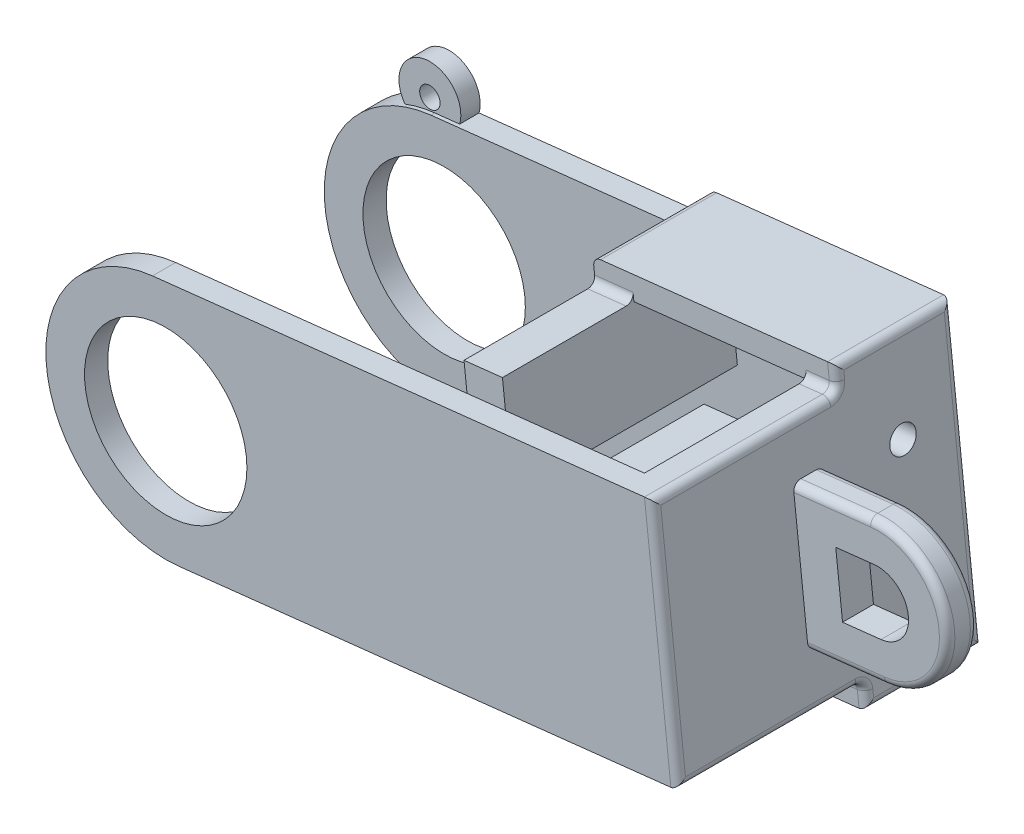
SolidWorks part; units mm, degrees
ref_plane "Front Plane" through (0, 0, 0) normal (0, 0, 1) x (1, 0, 0)
ref_plane "Top Plane" through (0, 0, 0) normal (0, 1, 0) x (1, 0, 0)
ref_plane "Right Plane" through (0, 0, 0) normal (1, 0, 0) x (0, 0, -1)
sketch "Sketch1" plane through (0, 0, 0) normal (0, 0, 1) x (1, 0, 0)
  line L0 (132.6238, -16.4902) -> (3.415, -30.8113)
  line L1 (132.6238, -16.4902) -> (125.7937, 45.1325)
  line L3 (125.7937, 45.1325) -> (-3.415, 30.8113)
  line L8 (33.2276, 36.08) -> (-40.322, 27.928) construction
  circle A0 centre (0, 0) radius 21
  arc A1 (-3.415, 30.8113) -> (3.415, -30.8113) centre (0, 0) ccw
  point P5 (71.547, -23.7484)
  dimension "D1" = 42
  dimension "D2" = 62
  dimension "D3" = 130
  dimension "D4" = 62
extrude "Boss-Extrude1" add sketch "Sketch1" against normal blind 6
sketch "Sketch2" plane through (0, 0, 0) normal (0, 0, 1) x (1, 0, 0)
  line L0 (125.7937, 45.1325) -> (132.6238, -16.4902)
  line L5 (132.6238, -16.4902) -> (125.7937, 45.1325) construction
  line L6 (132.6238, -16.4902) -> (124.6276, -17.3765)
  line L7 (3.415, -30.8113) -> (132.6238, -16.4902) construction
  line L8 (124.6276, -17.3765) -> (117.7975, 44.2462)
  line L9 (117.7975, 44.2462) -> (125.7937, 45.1325)
  dimension "D1" = 7.9962
extrude "Boss-Extrude2" add sketch "Sketch2" against normal blind 78
ref_plane "Plane1" through (0, 0, -39) normal (0, 0, 1) x (1, 0, 0)
sketch "Sketch3" plane through (0, 0, -6) normal (0, 0, -1) x (-1, 0, 0)
  circle A0 centre (-50, 5.8897) radius 3
  circle A1 centre (0, 0) radius 12.5 construction
  dimension "D1" = 6
  dimension "D2" = 50
extrude "Boss-Extrude3" add sketch "Sketch3" along normal blind 28
sketch "Sketch4" plane through (0, 0, -6) normal (0, 0, -1) x (-1, 0, 0)
  line L0 (-73.0714, 39.2889) -> (-79.9015, -22.3338)
  line L1 (-125.7937, 45.1325) -> (-117.7975, 44.2462) construction
  line L2 (-124.6276, -17.3765) -> (-132.6238, -16.4902) construction
  line L3 (-79.9015, -22.3338) -> (-69.9624, -23.4354)
  line L4 (-69.9624, -23.4354) -> (-63.1323, 38.1872)
  line L5 (-63.1323, 38.1872) -> (-73.0714, 39.2889)
  line L6 (-117.7975, 44.2462) -> (-124.6276, -17.3765) construction
  dimension "D1" = 10
  dimension "D2" = 45
extrude "Boss-Extrude4" add sketch "Sketch4" along normal blind 71
sketch "Sketch10" plane through (0, 0, -34) normal (0, 0, -1) x (-1, 0, 0)
  circle A0 centre (-50, 5.8897) radius 4
extrude "Boss-Extrude6" add sketch "Sketch10" against normal blind 1
mirror "Mirror1" about plane through (0, 0, -39) normal (0, 0, 1) of bodies 119 107
sketch "Sketch6" plane through (0, 0, -6) normal (0, 0, -1) x (-1, 0, 0)
  line L0 (-77.7989, 39.8128) -> (-50.5325, 36.7907)
  line L1 (-117.7975, 44.2462) -> (-73.0714, 39.2889) construction
  line L2 (-63.1323, 38.1872) -> (3.415, 30.8113) construction
  line L3 (-50.5325, 36.7907) -> (-51.8362, 25.0286)
  line L4 (-51.8362, 25.0286) -> (-77.7989, 27.9062)
  line L5 (-77.7989, 27.9062) -> (-77.7989, 39.8128)
extrude "Cut-Extrude1" cut sketch "Sketch6" along normal blind 8
ref_plane "Plane2" through (0, 0, 0) normal (-0.1102, 0.9939, 0) x (0.9939, 0.1102, 0)
mirror "Mirror4" about plane through (0, 0, 0) normal (-0.1102, 0.9939, 0) of "Cut-Extrude1"
sketch "Sketch8" plane through (66.5473, 7.3759, 0) normal (-0.9939, -0.1102, 0) x (0, 0, 1)
  line L0 (-72, -31) -> (-72, 31) construction
  line L1 (-72, 0) -> (-6, 0)
  line L2 (-72, 0) -> (-72, 6)
  line L3 (-72, 6) -> (-6, 6)
  line L4 (-6, 0) -> (-6, 6)
  line L5 (-6, 31) -> (-6, -31) construction
  dimension "D1" = 6
extrude "Cut-Extrude3" cut sketch "Sketch8" against normal blind 15
mirror "Mirror5" about plane through (81.456, 9.0284, -72) normal (0.1102, -0.9939, 0) of "Cut-Extrude3"
sketch "Sketch11" plane through (-3.415, 30.8113, 0) normal (-0.1102, 0.9939, 0) x (0.9939, 0.1102, 0)
  line L0 (66.9548, 72) -> (66.9548, 14) construction
  line L1 (130, 78) -> (66.9548, 78)
  line L2 (130, 78) -> (130, 48)
  line L3 (130, 48) -> (66.9548, 48)
  line L4 (66.9548, 78) -> (66.9548, 48)
  dimension "D1" = 30
extrude "Boss-Extrude7" add sketch "Sketch11" along normal blind 6
mirror "Mirror6" about plane through (0, 0, 0) normal (-0.1102, 0.9939, 0) of "Boss-Extrude7"
fillet "Fillet2" radius 2 14 edges at (125.7937, 45.1325, -24) (125.4632, 48.1142, -48) (125.1328, 51.0959, -63) (129.2088, 14.3211, -78) (133.2848, -22.4537, -63) (132.9543, -19.4719, -48) (132.6238, -16.4902, -24) (129.2088, 14.3211, 0) (70.6233, -29.3989, -63) (62.4713, 44.1507, -63) (68.1019, 38.7381, -48) (121.7956, 44.6893, -48) (74.9319, -22.8846, -48) (128.6257, -16.9333, -48)
sketch "Sketch12" plane through (129.2088, 14.3211, 0) normal (0.9939, 0.1102, 0) x (0, 0, -1)
  line L0 (50, -35) -> (76, -35) construction
  circle A0 centre (63, 14) radius 6.3103
  circle A1 centre (63, -16) radius 7.3998
  point P0 (63, 14)
  point P2 (63, -16)
  dimension "D1" = 30
  dimension "D2" = 19
hole_wizard "Tap Drill for M8 Tap1" positions "Sketch12" profile "Sketch13" hole size "M8" standard "GB"
sketch "Sketch13" plane through (127.6665, 28.2359, -63) normal (0, 0, 1) x (-0.1102, 0.9939, 0)
  line L0 (0, 0) -> (0, 22.0429)
  line L1 (0, 22.0429) -> (3.4, 20)
  line L2 (3.4, 20) -> (3.4, 0)
  line L5 (3.4, 0) -> (0, 0)
  line L10 (0, 22.0429) -> (-3.4, 20) construction
  line L11 (0, -6.35) -> (0, 107.95) construction
  dimension "孔直径" = 6.8
  dimension "孔深度" = 20
  dimension "导头角度" = 118
sketch "Sketch14" plane through (0, 0, -78) normal (0, 0, -1) x (-1, 0, 0)
  circle A0 centre (4.6836, 33.6759) radius 2.6393
  circle A1 centre (-4.6836, -33.6759) radius 2.75
  circle A2 centre (4.6836, 33.6759) radius 8
  circle A3 centre (-4.6836, -33.6759) radius 8
  dimension "D1" = 16
  dimension "D2" = 16
extrude "Boss-Extrude8" add sketch "Sketch14" against normal blind 5
sketch "Sketch15" plane through (129.2088, 14.3211, 0) normal (0.9939, 0.1102, 0) x (0, 0, -1)
  line L0 (42.9, 0) -> (-42.9, 0) construction
  line L1 (43, -18) -> (35, -18)
  line L2 (43, -18) -> (43, 18)
  line L3 (43, 18) -> (35, 18)
  line L4 (35, -18) -> (35, 18)
  line L5 (43, -18) -> (35, 18) construction
  line L6 (43, 18) -> (35, -18) construction
  line L7 (39, 41.8728) -> (39, -41.8728) construction
  point P0 (39, 0)
  dimension "D1" = 8
  dimension "D2" = 36
extrude "Boss-Extrude9" add sketch "Sketch15" along normal blind 20
sketch "Sketch16" plane through (0, 0, -43) normal (0, 0, -1) x (-1, 0, 0)
  line L0 (-151.07, -1.3661) -> (-147.1041, 34.4148) construction
  circle A0 centre (-149.087, 16.5244) radius 18
extrude "Boss-Extrude10" add sketch "Sketch16" against normal blind 8
sketch "Sketch17" plane through (0, 0, -43) normal (0, 0, -1) x (-1, 0, 0)
  line L6 (-138.2666, 23.3741) -> (-148.2057, 24.4757)
  line L7 (-149.9683, 8.5731) -> (-140.0292, 7.4714)
  line L8 (-140.0292, 7.4714) -> (-138.2666, 23.3741)
  line L9 (-138.2666, 23.3741) -> (-148.2057, 24.4757)
  line L10 (-149.9683, 8.5731) -> (-140.0292, 7.4714)
  line L11 (-140.0292, 7.4714) -> (-138.2666, 23.3741)
  arc A2 (-148.2057, 24.4757) -> (-149.9683, 8.5731) centre (-149.087, 16.5244) ccw
  arc A3 (-148.2057, 24.4757) -> (-149.9683, 8.5731) centre (-149.087, 16.5244) ccw
  dimension "D1" = 10
extrude "Cut-Extrude4" cut sketch "Sketch17" against normal blind 8
fillet "Fillet3" radius 2 6 edges at (137.165, 33.3132, -43) (141.1308, -2.4677, -43) (137.165, 33.3132, -35) (141.1308, -2.4677, -35) (166.9775, 18.5073, -35) (166.9775, 18.5073, -43)
